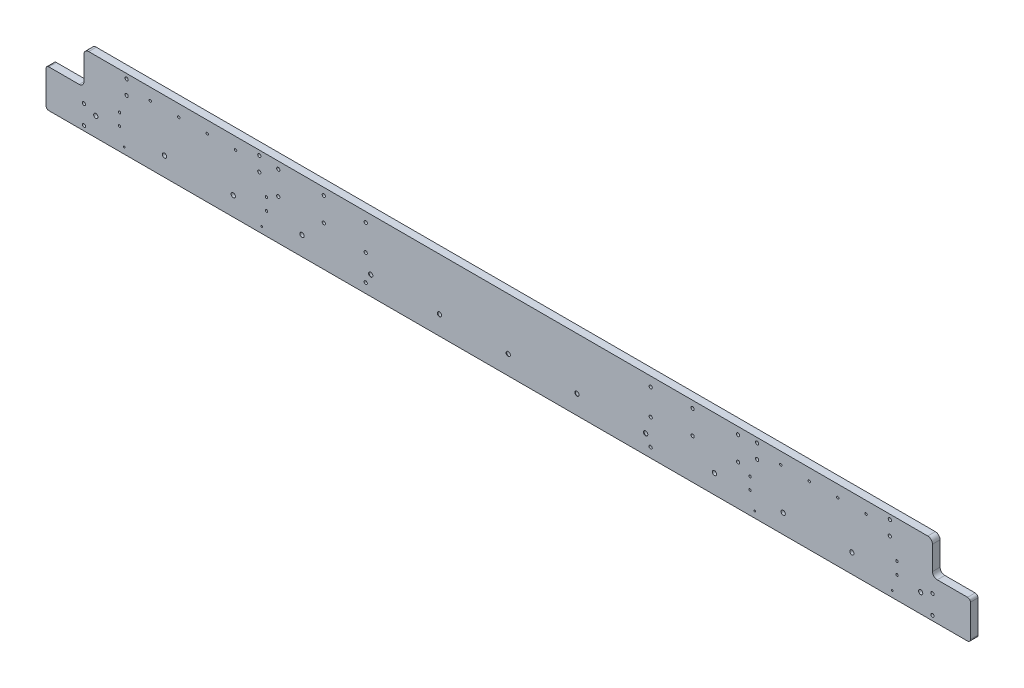
from build123d import *

# Parameters (mm, degrees)
SKETCH_6_W                     = 1950
SKETCH_6_H                     = 150
EXTRUDE_2_DEPTH                = 8
HOLE_WIZARD_M8_1_D             = 6.8
HOLE_WIZARD_M6_2_D             = 5
PATTERN_LINEAR_1_COUNT         = 4
PATTERN_LINEAR_1_PITCH         = 60
MIRROR_1_COPY_1_D              = 5
MIRROR_1_COPY_2_D              = 5
MIRROR_1_COPY_3_D              = 5
HOLE_WIZARD_M8_1_2_D           = 9
HOLE_WIZARD_M8_1_2_CBORE_D     = 15
HOLE_WIZARD_M8_1_2_CBORE_DEPTH = 9
PATTERN_LINEAR_3_COUNT         = 2
PATTERN_LINEAR_3_PITCH         = 145
PATTERN_LINEAR_4_COUNT         = 2
PATTERN_LINEAR_4_PITCH         = 435
HOLE_WIZARD_M8_2_D             = 9
HOLE_WIZARD_M8_2_CBORE_D       = 15
HOLE_WIZARD_M8_2_CBORE_DEPTH   = 15
PATTERN_LINEAR_5_COUNT         = 3
PATTERN_LINEAR_5_PITCH         = 145
MIRROR_4_COPY_1_D              = 9
MIRROR_4_COPY_1_CBORE_D        = 15
MIRROR_4_COPY_1_CBORE_DEPTH    = 9
MIRROR_4_COPY_2_D              = 9
MIRROR_4_COPY_2_CBORE_D        = 15
MIRROR_4_COPY_2_CBORE_DEPTH    = 15
MIRROR_4_COPY_3_D              = 9
MIRROR_4_COPY_3_CBORE_D        = 15
MIRROR_4_COPY_3_CBORE_DEPTH    = 15
SKETCH_29_W                    = 80
SKETCH_29_H                    = 70
CUT_EXTRUDE_1_DEPTH            = 979.011247379
HOLE_WIZARD_M8_6_D             = 6.8
PATTERN_LINEAR_6_COUNT         = 2
PATTERN_LINEAR_6_PITCH         = 145
FILLET_1_R                     = 6
HOLE_WIZARD_M6_1_D             = 5
FILLET_2_R                     = 10
FILLET_3_R                     = 10
HOLE_WIZARD_M8_7_D             = 6.8
HOLE_WIZARD_M8_8_D             = 6.8
HOLE_WIZARD_M4_1_D             = 3.3
HOLE_WIZARD_M4_2_D             = 3.3


with BuildPart() as part:
    # 草图6 → 凸台-拉伸2 (new, symmetric)
    with BuildSketch(Plane.XY):
        Rectangle(SKETCH_6_W, SKETCH_6_H)
    extrude(amount=EXTRUDE_2_DEPTH, both=True)

    # Hole Wizard M8 _1 (through all)
    with Locations(Plane.XY.offset(8)):
        with Locations((-805, 65), (-805, 35), (-525, 65), (-525, 35), (805, 35), (805, 65), (525, 35), (525, 65)):
            Hole(HOLE_WIZARD_M8_1_D / 2)

    # M6 螺纹孔2 (through all)
    with Locations(Plane.XY.offset(8)):
        with Locations((-575, 50)):
            hole_wizard_m6_2 = Hole(HOLE_WIZARD_M6_2_D / 2)

    # 阵列(线性)1: M6 螺纹孔2 ×4
    with Locations(*[(-i * PATTERN_LINEAR_1_PITCH, 0, 0) for i in range(1, PATTERN_LINEAR_1_COUNT)]):
        add(hole_wizard_m6_2, mode=Mode.SUBTRACT)

    # 镜向1: M6 螺纹孔2 across plane
    add(hole_wizard_m6_2.mirror(Plane(origin=(0, 0, 0), x_dir=(0, 0, 1), z_dir=(1, 0, 0))), mode=Mode.SUBTRACT)

    # 镜向1 copy 1 (through all)
    with Locations(Plane(origin=(60, 0, 8), x_dir=(-1, 0, 0), z_dir=(0, 0, 1))):
        with Locations((-575, -50)):
            Hole(MIRROR_1_COPY_1_D / 2)

    # 镜向1 copy 2 (through all)
    with Locations(Plane(origin=(120, 0, 8), x_dir=(-1, 0, 0), z_dir=(0, 0, 1))):
        with Locations((-575, -50)):
            Hole(MIRROR_1_COPY_2_D / 2)

    # 镜向1 copy 3 (through all)
    with Locations(Plane(origin=(180, 0, 8), x_dir=(-1, 0, 0), z_dir=(0, 0, 1))):
        with Locations((-575, -50)):
            Hole(MIRROR_1_COPY_3_D / 2)

    # Hole Wizard M8 _1 2 (through all)
    with Locations(Plane(origin=(0, 0, -8), x_dir=(-1, 0, 0), z_dir=(0, 0, -1))):
        with Locations((870, -35)):
            hole_wizard_m8_1_2 = CounterBoreHole(HOLE_WIZARD_M8_1_2_D / 2, HOLE_WIZARD_M8_1_2_CBORE_D / 2, HOLE_WIZARD_M8_1_2_CBORE_DEPTH)

    # 阵列(线性)3: Hole Wizard M8 _1 2 ×2
    with Locations(*[(i * PATTERN_LINEAR_3_PITCH, 0, 0) for i in range(1, PATTERN_LINEAR_3_COUNT)]):
        add(hole_wizard_m8_1_2, mode=Mode.SUBTRACT)

    # 阵列(线性)4: Hole Wizard M8 _1 2 ×2
    with Locations(*[(i * PATTERN_LINEAR_4_PITCH, 0, 0) for i in range(1, PATTERN_LINEAR_4_COUNT)]):
        add(hole_wizard_m8_1_2, mode=Mode.SUBTRACT)

    # M8 六角凹头螺钉的柱形沉头孔2 (through all)
    with Locations(Plane(origin=(0, 0, -8), x_dir=(-1, 0, 0), z_dir=(0, 0, -1))):
        with Locations((290, -35)):
            hole_wizard_m8_2 = CounterBoreHole(HOLE_WIZARD_M8_2_D / 2, HOLE_WIZARD_M8_2_CBORE_D / 2, HOLE_WIZARD_M8_2_CBORE_DEPTH)

    # 阵列(线性)5: M8 六角凹头螺钉的柱形沉头孔2 ×3
    with Locations(*[(i * PATTERN_LINEAR_5_PITCH, 0, 0) for i in range(1, PATTERN_LINEAR_5_COUNT)]):
        add(hole_wizard_m8_2, mode=Mode.SUBTRACT)

    # 镜向4: Hole Wizard M8 _1 2, M8 六角凹头螺钉的柱形沉头孔2 across plane
    add(hole_wizard_m8_1_2.mirror(Plane(origin=(0, 0, 0), x_dir=(0, 0, 1), z_dir=(1, 0, 0))), mode=Mode.SUBTRACT)
    add(hole_wizard_m8_2.mirror(Plane(origin=(0, 0, 0), x_dir=(0, 0, 1), z_dir=(1, 0, 0))), mode=Mode.SUBTRACT)

    # 镜向4 copy 1 (through all)
    with Locations(Plane(origin=(-435, 0, -8), x_dir=(1, 0, 0), z_dir=(0, 0, -1))):
        with Locations((870, 35)):
            CounterBoreHole(MIRROR_4_COPY_1_D / 2, MIRROR_4_COPY_1_CBORE_D / 2, MIRROR_4_COPY_1_CBORE_DEPTH)

    # 镜向4 copy 2 (through all)
    with Locations(Plane(origin=(-145, 0, -8), x_dir=(1, 0, 0), z_dir=(0, 0, -1))):
        with Locations((290, 35)):
            CounterBoreHole(MIRROR_4_COPY_2_D / 2, MIRROR_4_COPY_2_CBORE_D / 2, MIRROR_4_COPY_2_CBORE_DEPTH)

    # 镜向4 copy 3 (through all)
    with Locations(Plane(origin=(-290, 0, -8), x_dir=(1, 0, 0), z_dir=(0, 0, -1))):
        with Locations((290, 35)):
            CounterBoreHole(MIRROR_4_COPY_3_D / 2, MIRROR_4_COPY_3_CBORE_D / 2, MIRROR_4_COPY_3_CBORE_DEPTH)

    # 草图27 → M8 六角凹头螺钉的柱形沉头孔3 (revolve, cut)
    with BuildSketch(Plane(origin=(725, -35, -8), x_dir=(0, 1, 0), z_dir=(1, 0, 0))):
        Polygon((0, 0), (0, 26.453872786), (4.5, 23.75), (4.5, 8.6), (7, 8.6), (7, 0), align=None)
    hole_wizard_m8_3 = revolve(axis=Axis((725, -35, -14.35), (0, 0, 1)), mode=Mode.SUBTRACT)

    # 草图29 → 切除-拉伸1 (cut, through all)
    with BuildSketch(Plane(origin=(0, 0, -8), x_dir=(-1, 0, 0), z_dir=(0, 0, -1))):
        with Locations((-935, 40)):
            Rectangle(SKETCH_29_W, SKETCH_29_H)
    cut_extrude_1 = extrude(amount=-CUT_EXTRUDE_1_DEPTH, mode=Mode.SUBTRACT)

    # 镜向5: 切除-拉伸1 across plane
    add(cut_extrude_1.mirror(Plane(origin=(0, 0, 0), x_dir=(0, 0, 1), z_dir=(1, 0, 0))), mode=Mode.SUBTRACT)

    # M8 螺纹孔6 (through all)
    with Locations(Plane.XY.offset(8)):
        with Locations((-895, -65), (-895, -25)):
            hole_wizard_m8_6 = Hole(HOLE_WIZARD_M8_6_D / 2)

    # 镜向7: M8 螺纹孔6 across plane
    add(hole_wizard_m8_6.mirror(Plane(origin=(0, 0, 0), x_dir=(0, 0, 1), z_dir=(1, 0, 0))), mode=Mode.SUBTRACT)

    # 阵列(线性)6: M8 六角凹头螺钉的柱形沉头孔3 ×2
    with Locations(*[(-i * PATTERN_LINEAR_6_PITCH, 0, 0) for i in range(1, PATTERN_LINEAR_6_COUNT)]):
        add(hole_wizard_m8_3, mode=Mode.SUBTRACT)

    # 镜向8 copy 1 sketch → 镜向8 copy 1 (revolve, cut)
    with BuildSketch(Plane(origin=(-580, -35, -8), x_dir=(0, 1, 0), z_dir=(-1, 0, 0))):
        Polygon((0, 0), (0, -26.453872786), (4.5, -23.75), (4.5, -8.6), (7, -8.6), (7, 0), align=None)
    revolve(axis=Axis((-580, -35, -14.35), (0, 0, -1)), mode=Mode.SUBTRACT)

    # 镜向8 copy 2 sketch → 镜向8 copy 2 (revolve, cut)
    with BuildSketch(Plane(origin=(-725, -35, -8), x_dir=(0, 1, 0), z_dir=(-1, 0, 0))):
        Polygon((0, 0), (0, -26.453872786), (4.5, -23.75), (4.5, -8.6), (7, -8.6), (7, 0), align=None)
    revolve(axis=Axis((-725, -35, -14.35), (0, 0, -1)), mode=Mode.SUBTRACT)

    # 圆角1
    fillet_1_edges = [part.edges().sort_by_distance(p)[0] for p in [
        (975, 5, 0),
        (-975, 5, 0),
        (975, -75, 0),
        (-975, -75, 0),
    ]]
    fillet(fillet_1_edges, radius=FILLET_1_R)

    # M6 螺纹孔1 (through all)
    with Locations(Plane(origin=(0, 0, -8), x_dir=(-1, 0, 0), z_dir=(0, 0, -1))):
        with Locations((-820, -3.5), (-820, -28.5), (-510, -3.5), (-510, -28.5)):
            hole_wizard_m6_1 = Hole(HOLE_WIZARD_M6_1_D / 2)

    # 镜向9: M6 螺纹孔1 across plane
    add(hole_wizard_m6_1.mirror(Plane(origin=(0, 0, 0), x_dir=(0, 0, 1), z_dir=(1, 0, 0))), mode=Mode.SUBTRACT)

    # 圆角2
    fillet_2_edges = [part.edges().sort_by_distance(p)[0] for p in [
        (895, 5, 0),
        (-895, 5, 0),
    ]]
    fillet(fillet_2_edges, radius=FILLET_2_R)

    # 圆角3
    fillet_3_edges = [part.edges().sort_by_distance(p)[0] for p in [
        (895, 75, 0),
        (-895, 75, 0),
    ]]
    fillet(fillet_3_edges, radius=FILLET_3_R)

    # M8 螺纹孔7 (through all)
    with Locations(Plane(origin=(0, 0, -8), x_dir=(-1, 0, 0), z_dir=(0, 0, -1))):
        with Locations((-300.5, 55), (-300.5, 0), (-300.5, -55), (300.5, -55), (300.5, 0), (300.5, 55)):
            Hole(HOLE_WIZARD_M8_7_D / 2)

    # M8 螺纹孔8 (through all)
    with Locations(Plane(origin=(0, 0, -8), x_dir=(-1, 0, 0), z_dir=(0, 0, -1))):
        with Locations((-389, 60), (-389, 10), (-485, 10), (-485, 60), (485, 60), (485, 10), (389, 10), (389, 60)):
            Hole(HOLE_WIZARD_M8_8_D / 2)

    # M4 螺纹孔1 (through all)
    with Locations(Plane(origin=(0, 0, -8), x_dir=(-1, 0, 0), z_dir=(0, 0, -1))):
        with Locations((520, -62), (810, -62)):
            Hole(HOLE_WIZARD_M4_1_D / 2)

    # M4 螺纹孔2 (through all)
    with Locations(Plane(origin=(0, 0, -8), x_dir=(-1, 0, 0), z_dir=(0, 0, -1))):
        with Locations((-520, -62), (-810, -62)):
            Hole(HOLE_WIZARD_M4_2_D / 2)


solid = part.part
